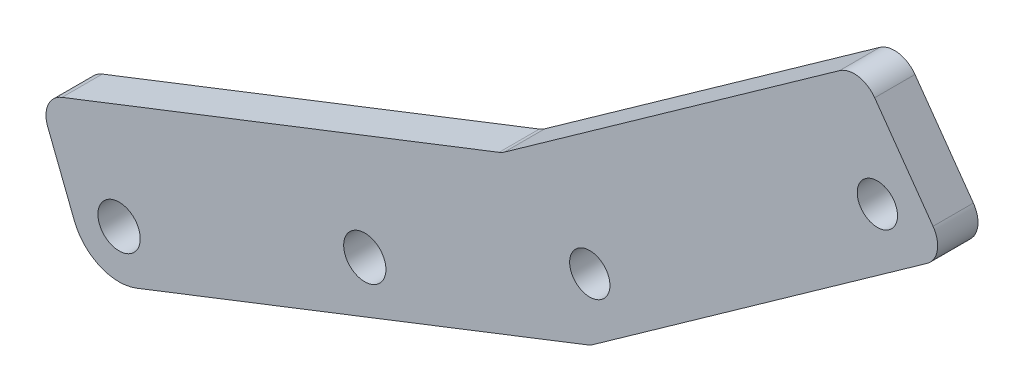
from build123d import *

# Parameters (mm, degrees)
SKETCH_1_R          = 4.191
SKETCH_1_R_2        = 4.2
EXTRUDE_1_DEPTH     = 8
SKETCH_2_R          = 4
CUT_EXTRUDE_1_DEPTH = 20


with BuildPart() as part:
    # 草图1 → 凸台-拉伸1 (new body)
    with BuildSketch(Plane.XY):
        with BuildLine():
            Line((87.979357684, 127.610653672), (-1.529435027, 92.60618121))
            ThreePointArc((-1.529435027, 92.60618121), (-8.81810924, 92.751332474), (-13.869342758, 98.007840879))
            Line((-13.869342758, 98.007840879), (-19.159529273, 111.53520395))
            ThreePointArc((-19.159529273, 111.53520395), (-19.083334383, 115.361279652), (-16.324012386, 118.012845804))
            Line((-16.324012386, 118.012845804), (70.420477634, 151.936274108))
            ThreePointArc((70.420477634, 151.936274108), (70.975789492, 152.193666623), (71.49549165, 152.516980454))
            Line((71.49549165, 152.516980454), (137.996231332, 199.768508694))
            ThreePointArc((137.996231332, 199.768508694), (141.726549955, 200.622548455), (144.968180855, 198.588712168))
            Line((144.968180855, 198.588712168), (156.55248685, 182.285220069))
            ThreePointArc((156.55248685, 182.285220069), (157.406526611, 178.554901446), (155.372690324, 175.313270545))
            Line((155.372690324, 175.313270545), (89.054371699, 128.191360017))
            ThreePointArc((89.054371699, 128.191360017), (88.534669542, 127.868046187), (87.979357684, 127.610653672))
        make_face()
        with Locations((43.76834518, 120.548384653)):
            Circle(SKETCH_1_R, mode=Mode.SUBTRACT)
        with Locations((-4.998559058, 101.47696491)):
            Circle(SKETCH_1_R_2, mode=Mode.SUBTRACT)
    extrude(amount=EXTRUDE_1_DEPTH)

    # 草图2 → 切除-拉伸1 (cut)
    with BuildSketch(Plane.XY.offset(8)):
        with Locations((145.504664302, 180.568940096)):
            Circle(SKETCH_2_R)
        with Locations((88.422593517, 140.051817853)):
            Circle(SKETCH_2_R)
    extrude(amount=-CUT_EXTRUDE_1_DEPTH, mode=Mode.SUBTRACT)


solid = part.part
